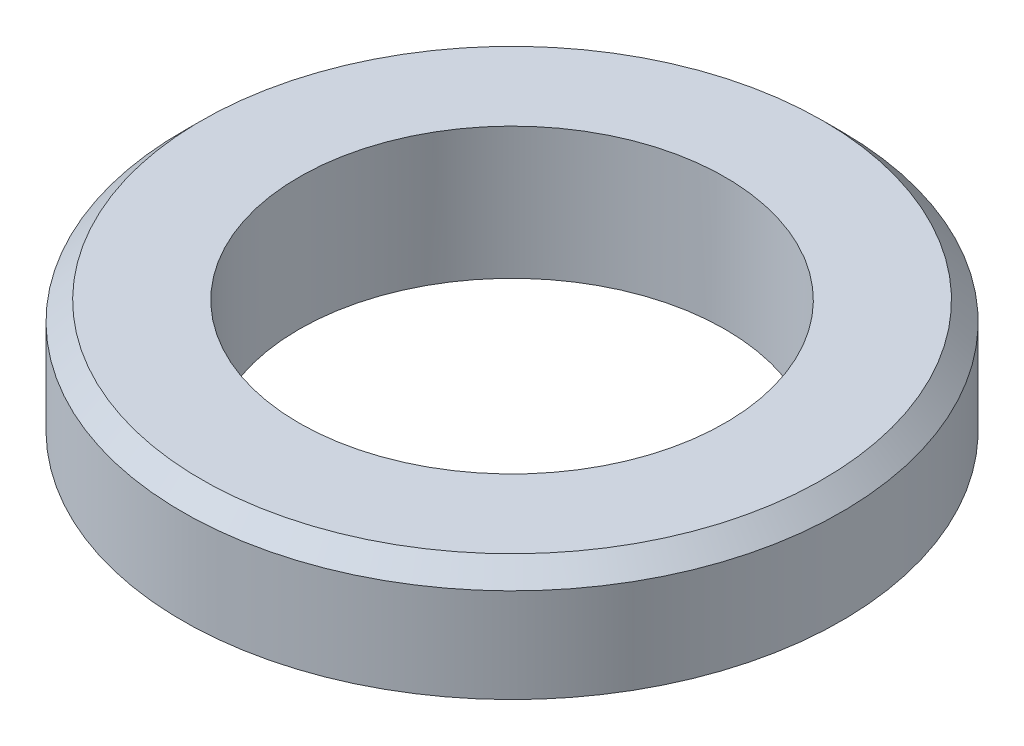
SolidWorks part; units mm, degrees
material "Q235B"
ref_plane "Front Plane" through (0, 0, 0) normal (0, 0, 1) x (1, 0, 0)
ref_plane "Top Plane" through (0, 0, 0) normal (0, 1, 0) x (1, 0, 0)
ref_plane "Right Plane" through (0, 0, 0) normal (1, 0, 0) x (0, 0, -1)
sketch "Sketch1" plane through (0, 0, 0) normal (1, 0, 0) x (0, 0, -1)
  line L0 (0, 0) -> (0, 14) construction
  line L1 (35, 12) -> (33, 14)
  line L2 (22.5, 0) -> (30, 0)
  line L3 (30, 0) -> (30, 2)
  line L4 (30, 2) -> (35, 2)
  line L5 (35, 2) -> (35, 12)
  line L6 (33, 14) -> (22.5, 14)
  line L7 (22.5, 14) -> (22.5, 0)
  point P3 (35, 14)
  dimension "D1" = 45
  dimension "D2" = 60
  dimension "D3" = 70
  dimension "D4" = 2
  dimension "D5" = 12
revolve "Revolve1" add sketch "Sketch1" angle 360 about L0
hole_wizard "G1-1/2 Tapped Hole1" positions "Sketch2" profile "Sketch3" tap size "G1-1/2" standard "GB"
sketch "Sketch2" plane through (0, 14, 0) normal (0, 1, 0) x (1, 0, 0)
  point P0 (0, 0)
sketch "Sketch3" plane through (0, 14, 0) normal (1, 0, 0) x (0, 0, 1)
  line L0 (0, 0) -> (0, 116.1345)
  line L1 (0, 116.1345) -> (22.625, 102.54)
  line L2 (22.625, 102.54) -> (22.625, 0)
  line L5 (22.625, 0) -> (0, 0)
  line L10 (0, 116.1345) -> (-22.625, 102.54) construction
  line L11 (0, -6.35) -> (0, 107.95) construction
  dimension "螺纹孔钻头直径" = 45.25
  dimension "螺纹孔钻头深度" = 102.54
  dimension "导头角度" = 118
cosmetic thread "Hole Cosmetic Thread1"
